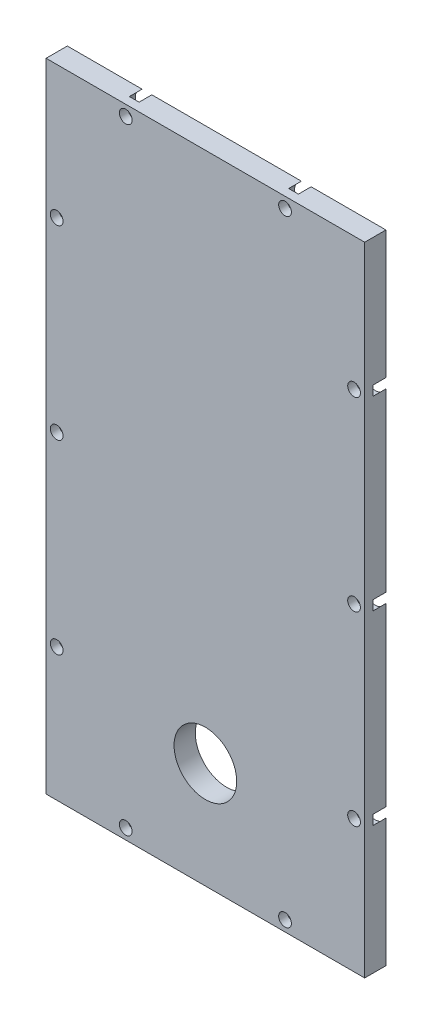
SolidWorks part; units mm, degrees
material "6061Al"
ref_plane "前视基准面" through (0, 0, 0) normal (0, 0, 1) x (1, 0, 0)
ref_plane "上视基准面" through (0, 0, 0) normal (0, 1, 0) x (1, 0, 0)
ref_plane "右视基准面" through (0, 0, 0) normal (1, 0, 0) x (0, 0, -1)
sketch "草图1" plane through (0, 0, 0) normal (0, 0, 1) x (1, 0, 0)
  line L1 (-30, -60) -> (30, -60)
  line L2 (-30, -60) -> (-30, 60)
  line L3 (-30, 60) -> (30, 60)
  line L4 (30, -60) -> (30, 60)
  line L5 (-30, -60) -> (30, 60) construction
  line L6 (-30, 60) -> (30, -60) construction
  point P0 (0, 0)
  dimension "D1" = 120
  dimension "D2" = 60
extrude "凸台-拉伸1" add sketch "草图1" along normal mid plane 4
hole_wizard "M2 六角凹头螺钉的柱形沉头孔1" positions "草图4" profile "草图5" counterbore size "M2" standard "ISO" end condition through all
sketch "草图4" plane through (0, 0, -2) normal (0, 0, -1) x (-1, 0, 0)
  line L12 (-28, 58) -> (-28, -58)
  line L13 (-28, -58) -> (28, -58)
  line L14 (28, -58) -> (28, 58)
  line L15 (28, 58) -> (-28, 58)
  line L16 (-28, 58) -> (-28, -58)
  line L17 (-28, -58) -> (28, -58)
  line L18 (28, -58) -> (28, 58)
  point P35 (-28, 0)
  point P41 (28, 0)
  point P43 (-15, 58)
  point P46 (15, 58)
  point P49 (-28, 35)
  point P52 (28, 35)
  point P55 (-28, -35)
  point P58 (-28, -35)
  point P60 (28, -35)
  point P63 (15, -58)
  point P66 (-15, -58)
  dimension "D1" = 2
sketch "草图5" plane through (15, -58, -2) normal (1, 0, 0) x (0, 1, 0)
  line L0 (0, 0) -> (0, 4)
  line L1 (0, 4) -> (1.2, 4)
  line L3 (1.2, 4) -> (1.2, 2.4)
  line L4 (1.2, 2.4) -> (2.2, 2.4)
  line L5 (2.2, 2.4) -> (2.2, 0)
  line L7 (2.2, 0) -> (0, 0)
  line L11 (0, -6.35) -> (0, 107.95) construction
  dimension "通孔孔直径" = 2.4
  dimension "通孔孔深度" = 4
  dimension "柱形沉头孔直径" = 4.4
  dimension "柱形沉头孔深度" = 2.4
sketch "草图7" plane through (0, 0, -2) normal (0, 0, -1) x (-1, 0, 0)
  line L1 (14.0835, -60) -> (-14.0835, -60) construction
  circle A0 centre (0, -40) radius 5.9
  dimension "D1" = 11.8
  dimension "D2" = 20
extrude "切除-拉伸2" cut sketch "草图7" against normal through all
